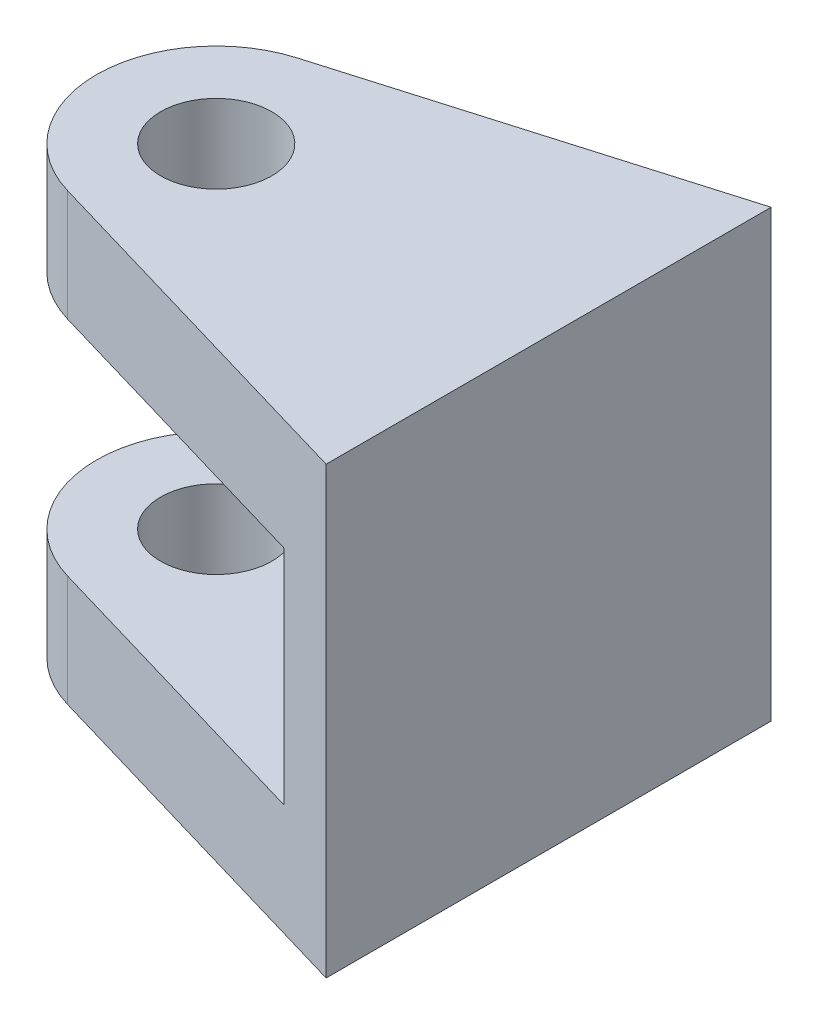
from build123d import *

# Parameters (mm, degrees)
BOSS_EXTRUDE1_DEPTH = 40
CUT_EXTRUDE1_DEPTH  = 20
SKETCH3_R           = 5
CUT_EXTRUDE2_DEPTH  = 70


with BuildPart() as part:
    # Sketch1 → Boss-Extrude1 (new body)
    with BuildSketch(Plane(origin=(0, 0, 0), x_dir=(1, 0, 0), z_dir=(0, 1, 0))):
        with BuildLine():
            Line((0, 0), (0, -40))
            Line((0, -40), (-32.916811342, -30.326541582))
            ThreePointArc((-32.916811342, -30.326541582), (-40.645313725, -20), (-32.916811342, -9.673458418))
            Line((-32.916811342, -9.673458418), (0, 0))
        make_face()
    extrude(amount=BOSS_EXTRUDE1_DEPTH)

    # Sketch2 → Cut-Extrude1 (cut)
    with BuildSketch(Plane(origin=(0, 10, 0), x_dir=(-1, 0, 0), z_dir=(0, -1, 0))):
        with BuildLine():
            Line((5.381519546, -1.581499041), (5.381519546, -38.418500959))
            Line((5.381519546, -38.418500959), (32.916811342, -30.326541582))
            ThreePointArc((32.916811342, -30.326541582), (40.645313725, -20), (32.916811342, -9.673458418))
            Line((32.916811342, -9.673458418), (5.381519546, -1.581499041))
        make_face()
    extrude(amount=-CUT_EXTRUDE1_DEPTH, mode=Mode.SUBTRACT)

    # Sketch3 → Cut-Extrude2 (cut, symmetric)
    with BuildSketch(Plane(origin=(0, 10, 0), x_dir=(-1, 0, 0), z_dir=(0, -1, 0))):
        with Locations(Location((29.882089371, -20, 0), (0, 0, 90))):
            Circle(SKETCH3_R)
    extrude(amount=CUT_EXTRUDE2_DEPTH, both=True, mode=Mode.SUBTRACT)


solid = part.part
